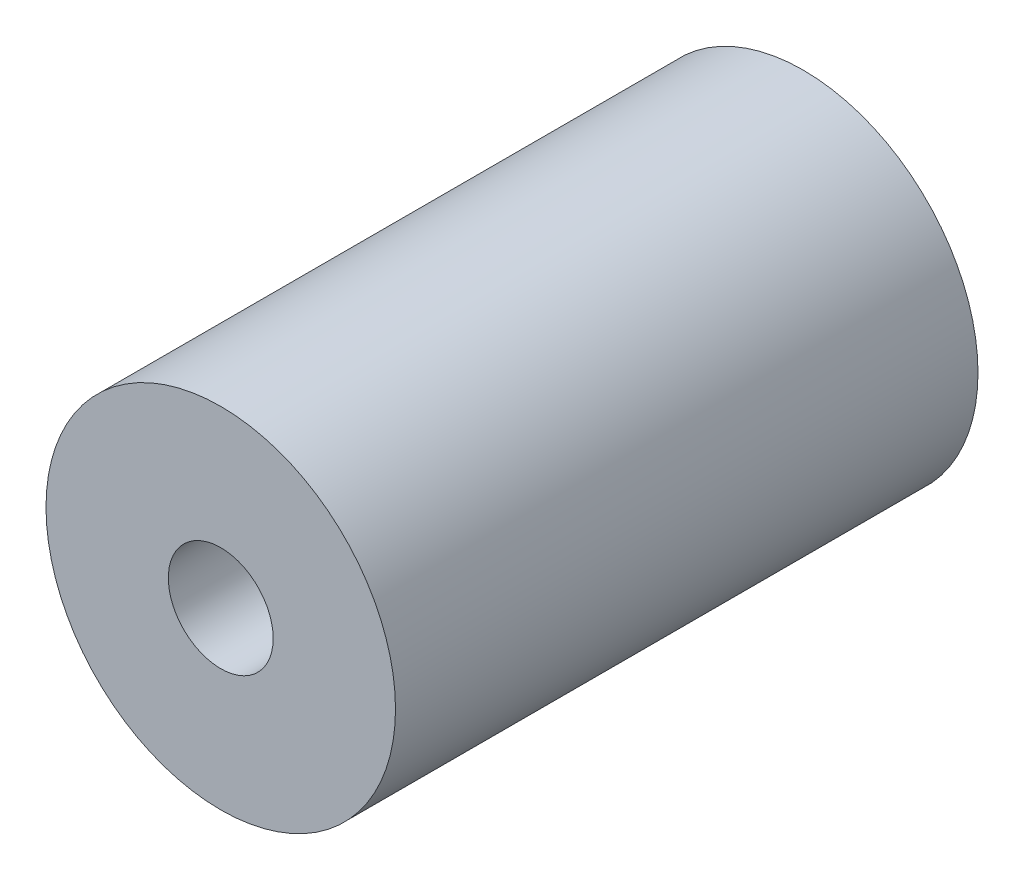
SolidWorks part; units mm, degrees
material "1023 碳钢板 (SS)"
ref_plane "前视基准面" through (0, 0, 0) normal (0, 0, 1) x (1, 0, 0)
ref_plane "上视基准面" through (0, 0, 0) normal (0, 1, 0) x (1, 0, 0)
ref_plane "右视基准面" through (0, 0, 0) normal (1, 0, 0) x (0, 0, -1)
sketch "草图1" plane through (0, 0, 0) normal (0, 0, 1) x (1, 0, 0)
  circle A0 centre (0, 0) radius 15
  circle A1 centre (0, 0) radius 4.5
  dimension "D1" = 30
  dimension "D2" = 9
extrude "凸台-拉伸1" add sketch "草图1" along normal blind 50 contours A1 | A0
